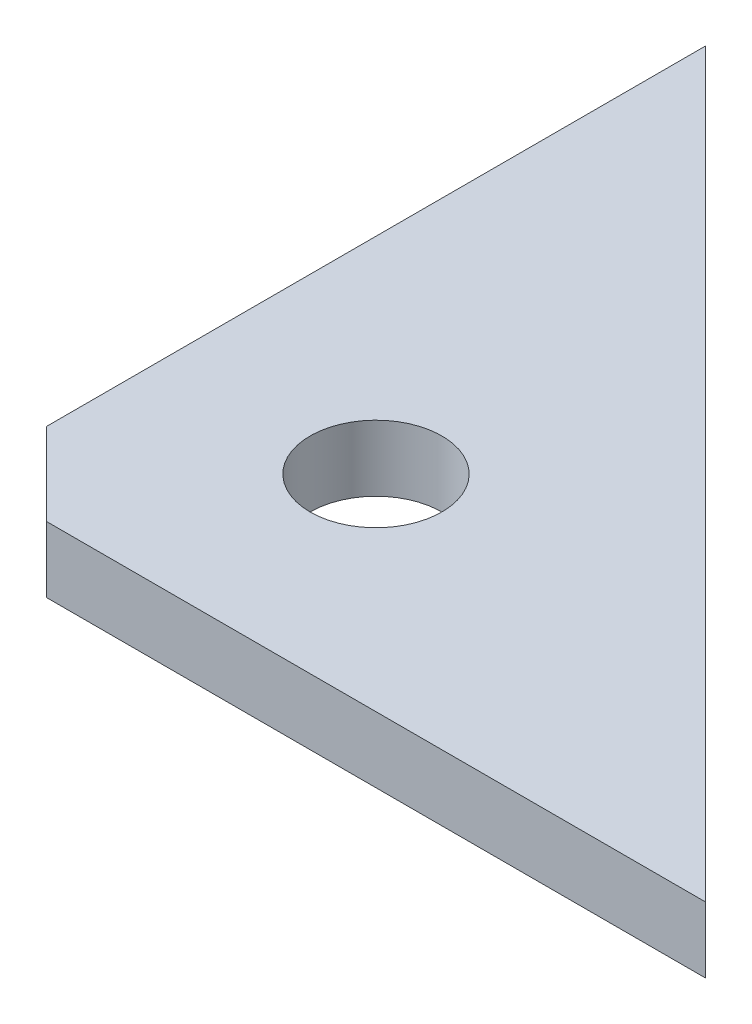
SolidWorks part; units mm, degrees
material "Q235"
ref_plane "前视基准面" through (0, 0, 0) normal (0, 0, 1) x (1, 0, 0)
ref_plane "上视基准面" through (0, 0, 0) normal (0, 1, 0) x (1, 0, 0)
ref_plane "右视基准面" through (0, 0, 0) normal (1, 0, 0) x (0, 0, -1)
sketch "草图1" plane through (0, 0, 0) normal (0, 1, 0) x (1, 0, 0)
  line L0 (0, 0) -> (0, 90)
  line L1 (0, 90) -> (90, 0)
  line L2 (90, 0) -> (0, 0)
  dimension "D1" = 90
  dimension "D2" = 90
extrude "凸台-拉伸1" add sketch "草图1" along normal blind 8
chamfer "倒角1" distance 10 angle 45 1 edges at (0, 4, 0)
hole_wizard "Ø16.0 (16) 直径孔1" positions "草图3" profile "草图2" hole size "Ø16.0" standard "Gb" end condition through all
sketch "草图3" plane through (0, 8, 0) normal (0, 1, 0) x (1, 0, 0)
  line L0 (10, 0) -> (90, 0) construction
  line L1 (0, 90) -> (0, 10) construction
  point P0 (25, 25)
  dimension "D1" = 25
  dimension "D2" = 25
sketch "草图2" plane through (25, 8, -25) normal (1, 0, 0) x (0, 0, 1)
  line L0 (0, 0) -> (0, 8)
  line L1 (0, 8) -> (8, 8)
  line L2 (8, 8) -> (8, 0)
  line L5 (8, 0) -> (0, 0)
  line L11 (0, -6.35) -> (0, 107.95) construction
  dimension "通孔孔直径" = 16
  dimension "通孔孔深度" = 8
